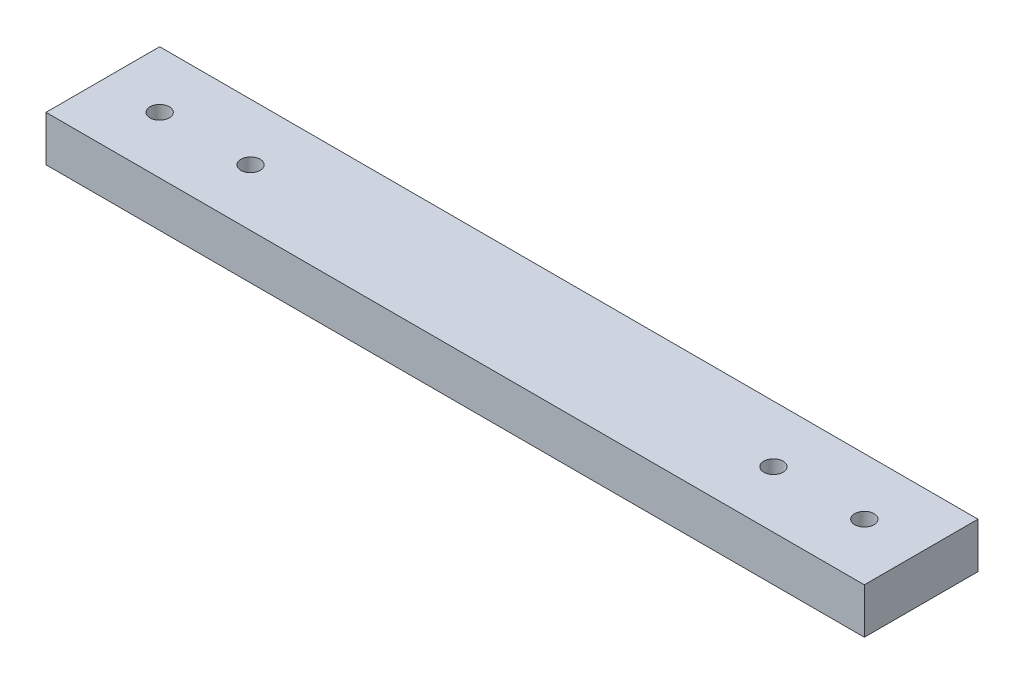
from build123d import *

# Parameters (mm, degrees)
SKETCH_1_W          = 360
SKETCH_1_H          = 50
SKETCH_1_R          = 2.5
EXTRUDE_1_DEPTH     = 20
HOLE_WIZARD_M10_1_D = 8.5


with BuildPart() as part:
    # 草图1 → 凸台-拉伸1 (new body)
    with BuildSketch(Plane.XZ.offset(-47)):
        with Locations((180, -25)):
            Rectangle(SKETCH_1_W, SKETCH_1_H)
        with Locations(Location((335, -25, 0), (0, 0, 90))):
            Circle(SKETCH_1_R, mode=Mode.SUBTRACT)
        with Locations(Location((65, -25, 0), (0, 0, 90))):
            Circle(SKETCH_1_R, mode=Mode.SUBTRACT)
        with Locations(Location((25, -25, 0), (0, 0, 90))):
            Circle(SKETCH_1_R, mode=Mode.SUBTRACT)
        with Locations(Location((295, -25, 0), (0, 0, 90))):
            Circle(SKETCH_1_R, mode=Mode.SUBTRACT)
    extrude(amount=-EXTRUDE_1_DEPTH)

    # M10 螺纹孔1 (through all)
    with Locations(Plane(origin=(0, 47, 0), x_dir=(-1, 0, 0), z_dir=(0, -1, 0))):
        with Locations((-335, 25), (-295, 25), (-65, 25), (-25, 25)):
            Hole(HOLE_WIZARD_M10_1_D / 2)


solid = part.part
